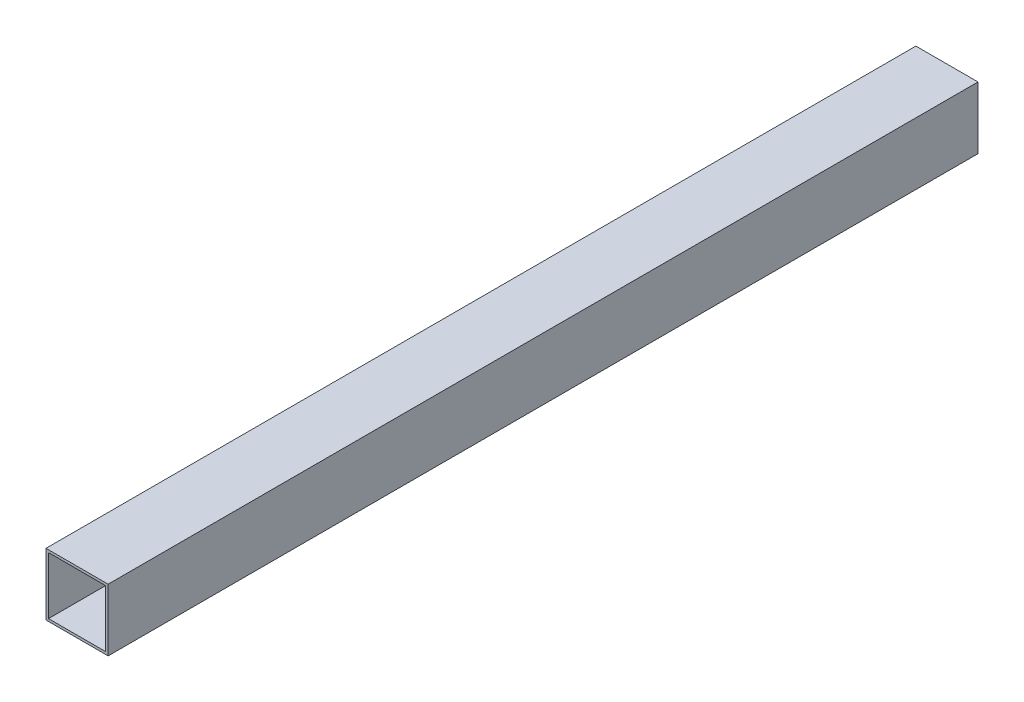
from build123d import *

# Parameters (mm, degrees)
SKETCH1_W           = 50
SKETCH1_H           = 50
SKETCH1_W_2         = 46
SKETCH1_H_2         = 46
BOSS_EXTRUDE1_DEPTH = 700


with BuildPart() as part:
    # Sketch1 → Boss-Extrude1 (new body)
    with BuildSketch(Plane.XY):
        Rectangle(SKETCH1_W, SKETCH1_H)
        Rectangle(SKETCH1_W_2, SKETCH1_H_2, mode=Mode.SUBTRACT)
    extrude(amount=BOSS_EXTRUDE1_DEPTH)


solid = part.part
